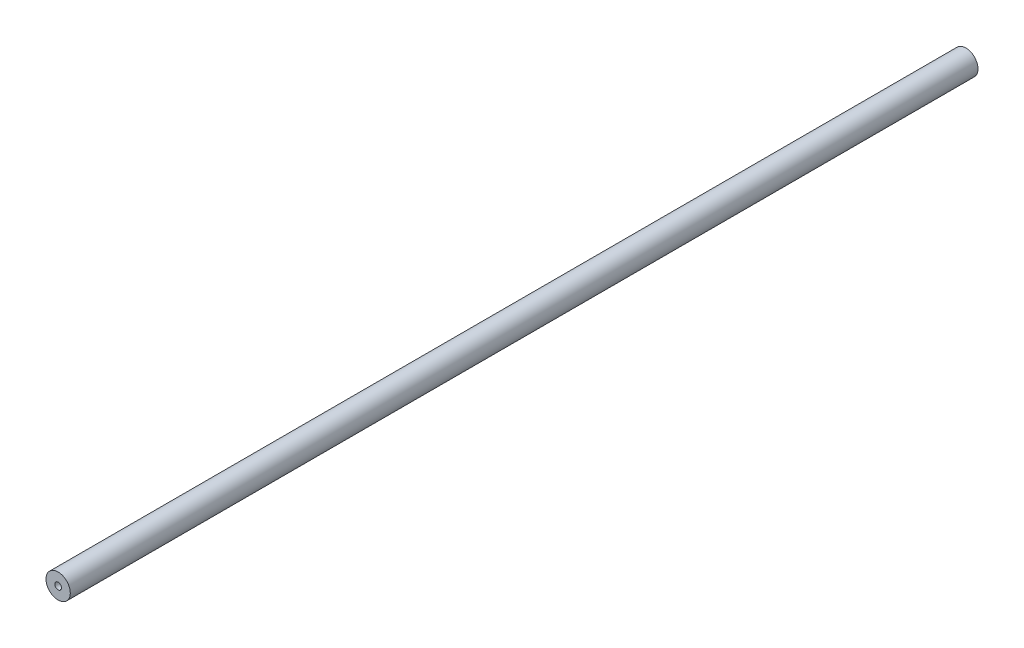
from build123d import *

# Parameters (mm, degrees)
SKETCH_1_R             = 6
EXTRUDE_1_DEPTH        = 448
HOLE_WIZARD_M4_1_D     = 3.3
HOLE_WIZARD_M4_1_DEPTH = 15
HOLE_WIZARD_M4_1_TIP   = 0.991420021
HOLE_WIZARD_M4_2_D     = 3.3
HOLE_WIZARD_M4_2_DEPTH = 15
HOLE_WIZARD_M4_2_TIP   = 0.991420021


with BuildPart() as part:
    # 草图1 → 凸台-拉伸1 (new body)
    with BuildSketch(Plane.XY):
        Circle(SKETCH_1_R)
    extrude(amount=EXTRUDE_1_DEPTH)

    # M4 螺纹孔1
    with Locations(Plane(origin=(0, 0, 0), x_dir=(-1, 0, 0), z_dir=(0, 0, -1))):
        with Locations((0, 0)):
            Hole(HOLE_WIZARD_M4_1_D / 2, depth=HOLE_WIZARD_M4_1_DEPTH)
            with Locations((0, 0, -(HOLE_WIZARD_M4_1_DEPTH + HOLE_WIZARD_M4_1_TIP / 2))):  # 118° drill point
                Cone(0, HOLE_WIZARD_M4_1_D / 2, HOLE_WIZARD_M4_1_TIP, mode=Mode.SUBTRACT)

    # M4 螺纹孔2
    with Locations(Plane.XY.offset(448)):
        with Locations((0, 0)):
            Hole(HOLE_WIZARD_M4_2_D / 2, depth=HOLE_WIZARD_M4_2_DEPTH)
            with Locations((0, 0, -(HOLE_WIZARD_M4_2_DEPTH + HOLE_WIZARD_M4_2_TIP / 2))):  # 118° drill point
                Cone(0, HOLE_WIZARD_M4_2_D / 2, HOLE_WIZARD_M4_2_TIP, mode=Mode.SUBTRACT)


solid = part.part
